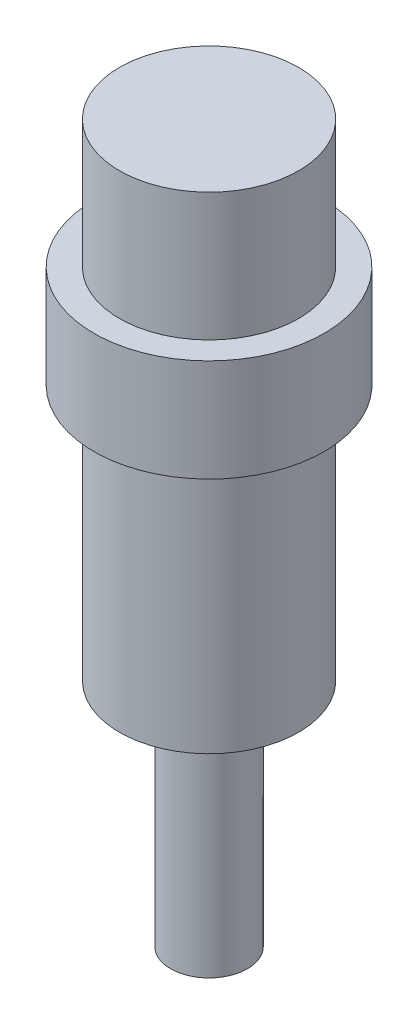
SolidWorks part; units mm, degrees
ref_plane "前视基准面" through (0, 0, 0) normal (0, 0, 1) x (1, 0, 0)
ref_plane "上视基准面" through (0, 0, 0) normal (0, 1, 0) x (1, 0, 0)
ref_plane "右视基准面" through (0, 0, 0) normal (1, 0, 0) x (0, 0, -1)
sketch "草图3" plane through (0, 0, 0) normal (0, 0, 1) x (1, 0, 0)
  line L0 (0, 0) -> (0, 9076.3779) construction
  line L1 (0, 10.0707) -> (3.5, 10.0707)
  line L2 (3.5, 10.0707) -> (3.5, 5.0707)
  line L3 (3.5, 5.0707) -> (4.5, 5.0707)
  line L4 (4.5, 5.0707) -> (4.5, 1.0707)
  line L5 (4.5, 1.0707) -> (3.5, 1.0707)
  line L6 (3.5, 1.0707) -> (3.5, -8.9293)
  line L7 (3.5, -8.9293) -> (1.5, -8.9293)
  line L8 (1.5, -8.9293) -> (1.5, -17.9293)
  line L9 (1.5, -17.9293) -> (0, -17.9293)
  line L10 (0, 10.0707) -> (0, -17.9293)
  dimension "D1" = 3.5
  dimension "D2" = 5
  dimension "D3" = 1
  dimension "D4" = 4
  dimension "D5" = 1
  dimension "D6" = 10
  dimension "D7" = 1.5
  dimension "D8" = 9
revolve "旋转19" add sketch "草图3" angle 360 about L0
